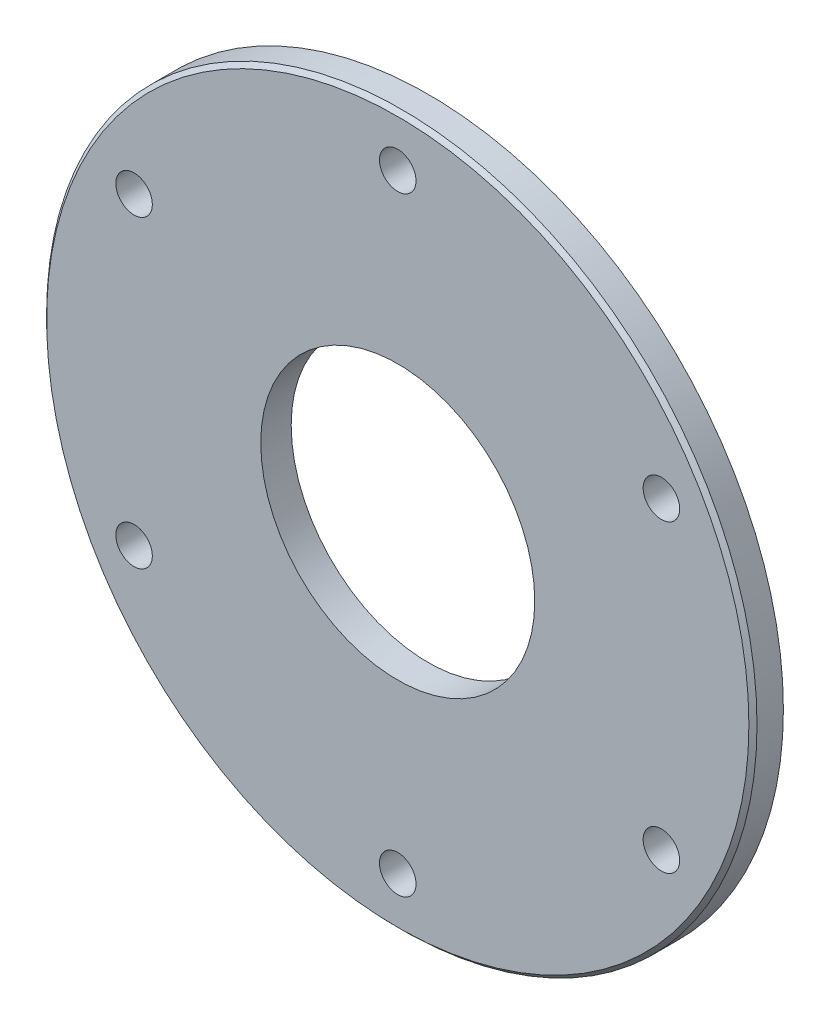
from build123d import *

# Parameters (mm, degrees)
SKETCH1_R           = 125
SKETCH1_R_2         = 110
BOSS_EXTRUDE1_DEPTH = 18
SKETCH2_R           = 175
SKETCH2_R_2         = 9
BOSS_EXTRUDE2_DEPTH = 15
CHAMFER1_SIZE       = 2
SKETCH3_R           = 67.5
CUT_EXTRUDE1_DEPTH  = 250.677792364


with BuildPart() as part:
    # Sketch1 → Boss-Extrude1 (new body)
    with BuildSketch(Plane.XY):
        with Locations(Location((0, 0, 0), (0, 0, 180))):
            Circle(SKETCH1_R)
        with Locations(Location((0, 0, 0), (0, 0, 180))):
            Circle(SKETCH1_R_2, mode=Mode.SUBTRACT)
    extrude(amount=BOSS_EXTRUDE1_DEPTH)

    # Sketch2 → Boss-Extrude2 (add)
    with BuildSketch(Plane.XY.offset(18)):
        Circle(SKETCH2_R)
        with Locations((0, 150)):
            Circle(SKETCH2_R_2, mode=Mode.SUBTRACT)
        with Locations((-129.903810568, 75)):
            Circle(SKETCH2_R_2, mode=Mode.SUBTRACT)
        with Locations((-129.903810568, -75)):
            Circle(SKETCH2_R_2, mode=Mode.SUBTRACT)
        with Locations((0, -150)):
            Circle(SKETCH2_R_2, mode=Mode.SUBTRACT)
        with Locations((129.903810568, -75)):
            Circle(SKETCH2_R_2, mode=Mode.SUBTRACT)
        with Locations((129.903810568, 75)):
            Circle(SKETCH2_R_2, mode=Mode.SUBTRACT)
    extrude(amount=BOSS_EXTRUDE2_DEPTH)

    # Chamfer1
    chamfer1_edges = [part.edges().sort_by_distance(p)[0] for p in [
        (-175, 0, 33),
    ]]
    chamfer(chamfer1_edges, length=CHAMFER1_SIZE)

    # Sketch3 → Cut-Extrude1 (cut, through all)
    with BuildSketch(Plane.XY.offset(33)):
        Circle(SKETCH3_R)
    extrude(amount=-CUT_EXTRUDE1_DEPTH, mode=Mode.SUBTRACT)


solid = part.part
